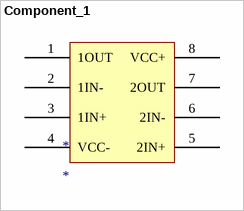
[diagram p0: symbol Component_1]
# Altium schematic symbol library MISC89340-11.SchLib: 1 symbol
Pins are listed as number, name and electrical type; pins without a type are passive.


## Component_1
designator *
footprint NE5532
pins: 1 1OUT, 2 1IN-, 3 1IN+, 4 VCC-, 5 2IN+, 6 2IN-, 7 2OUT, 8 VCC+